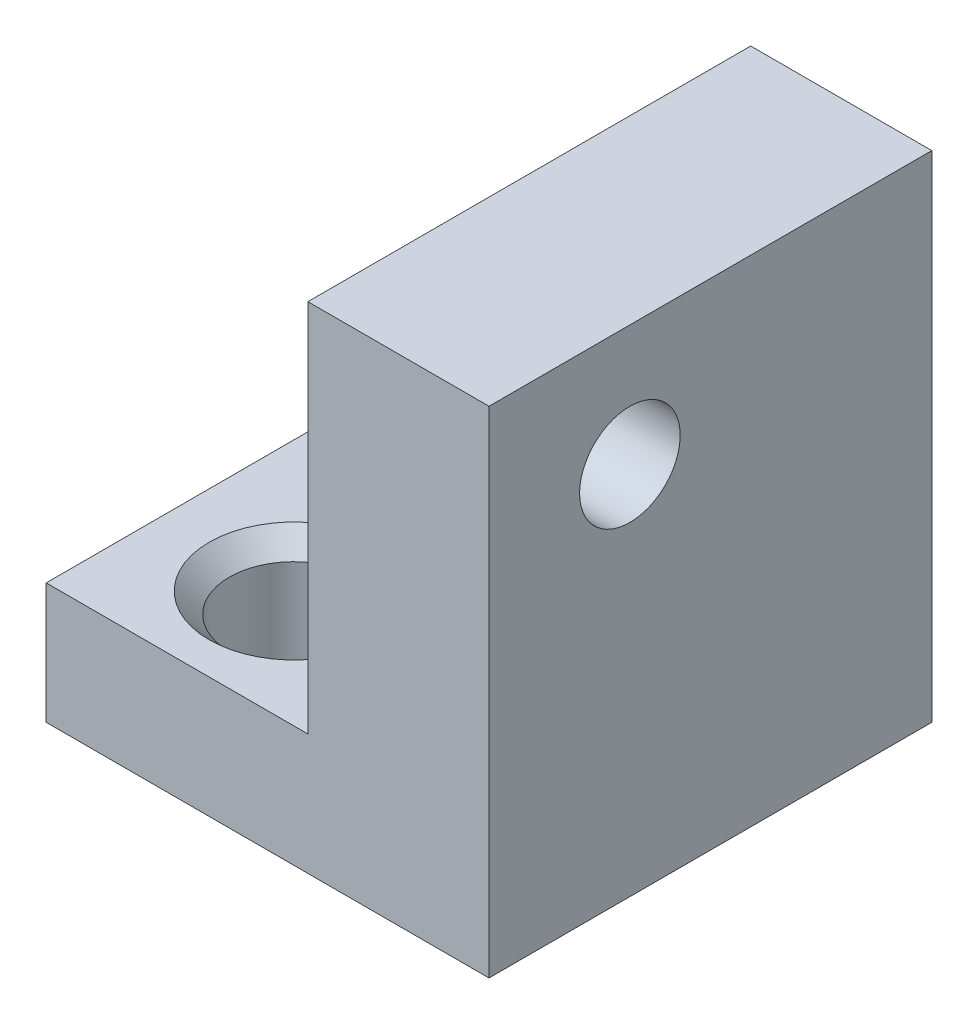
SolidWorks part; units mm, degrees
ref_plane "Front Plane" through (0, 0, 0) normal (0, 0, 1) x (1, 0, 0)
ref_plane "Top Plane" through (0, 0, 0) normal (0, 1, 0) x (1, 0, 0)
ref_plane "Right Plane" through (0, 0, 0) normal (1, 0, 0) x (0, 0, -1)
sketch "Sketch1" plane through (0, 0, 0) normal (0, 1, 0) x (1, 0, 0)
  line L1 (-5.5, 5.5) -> (5.5, 5.5)
  line L2 (-5.5, 5.5) -> (-5.5, -5.5)
  line L3 (-5.5, -5.5) -> (5.5, -5.5)
  line L4 (5.5, 5.5) -> (5.5, -5.5)
  line L5 (-5.5, 5.5) -> (5.5, -5.5) construction
  line L6 (-5.5, -5.5) -> (5.5, 5.5) construction
  point P0 (0, 0)
  dimension "D1" = 11
  dimension "D2" = 11
extrude "Boss-Extrude1" add sketch "Sketch1" along normal blind 3
sketch "Sketch2" plane through (0, 3, 0) normal (0, 1, 0) x (1, 0, 0)
  line L1 (5.5, 5.5) -> (1, 5.5)
  line L2 (5.5, 5.5) -> (5.5, -5.5)
  line L3 (5.5, -5.5) -> (1, -5.5)
  line L4 (1, 5.5) -> (1, -5.5)
  dimension "D1" = 4.5
  dimension "D2" = 11
extrude "Boss-Extrude2" add sketch "Sketch2" along normal blind 9.3
hole_wizard "M3 Tapped Hole1" positions "Sketch3" profile "Sketch4" tap size "M3" standard "GB"
sketch "Sketch3" plane through (1, 0, 0) normal (-1, 0, 0) x (0, 0, 1)
  line L0 (-5.5, 12.3) -> (5.5, 12.3) construction
  line L1 (5.5, 12.3) -> (5.5, 3) construction
  point P0 (2, 9.3)
  dimension "D1" = 3
  dimension "D2" = 3.5
sketch "Sketch4" plane through (1, 9.3, 2) normal (0, 1, 0) x (0, 0, 1)
  line L0 (0, 0) -> (0, 9.2511)
  line L1 (0, 9.2511) -> (1.25, 8.5)
  line L2 (1.25, 8.5) -> (1.25, 0)
  line L5 (1.25, 0) -> (0, 0)
  line L10 (0, 9.2511) -> (-1.25, 8.5) construction
  line L11 (0, -6.35) -> (0, 107.95) construction
  dimension "螺纹孔钻头直径" = 2.5
  dimension "螺纹孔钻头深度" = 8.5
  dimension "导头角度" = 118
cosmetic thread "Hole Thread 1" parameters "D1"=4, "D2"=3
sketch "Sketch5" plane through (0, 3, 0) normal (0, 1, 0) x (1, 0, 0)
  line L0 (-5.5, 5.5) -> (-5.5, -5.5) construction
  line L1 (1, 5.5) -> (-5.5, 5.5) construction
  line L2 (-5.5, -5.5) -> (1, -5.5) construction
  circle A0 centre (-2.25, 2.6) radius 1.6
  circle A1 centre (-2.25, -2.6) radius 1.6
  dimension "D1" = 3.25
  dimension "D2" = 2.9
  dimension "D3" = 3.25
  dimension "D4" = 2.9
extrude "Cut-Extrude1" cut sketch "Sketch5" against normal through all
chamfer "Chamfer1" distance 0.5 angle 45 2 edges at (-2.25, 3, 4.2) (-2.25, 3, -1)
